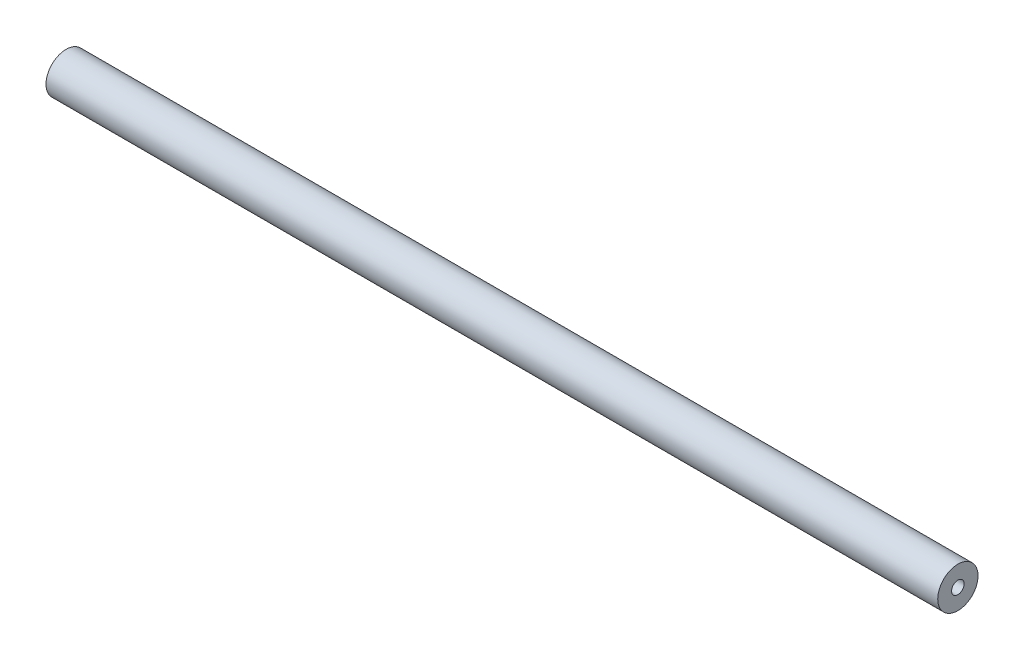
SolidWorks part; units mm, degrees
material "45"
ref_plane "Front" through (0, 0, 0) normal (0, 0, 1) x (1, 0, 0)
ref_plane "Top" through (0, 0, 0) normal (0, 1, 0) x (1, 0, 0)
ref_plane "Right" through (0, 0, 0) normal (1, 0, 0) x (0, 0, -1)
sketch "Sketch1" plane through (0, 0, 0) normal (0, 0, 1) x (1, 0, 0)
  line L0 (0, 0) -> (-177, 0) construction
  line L2 (177, 8) -> (-177, 8)
  line L6 (-177, 8) -> (-177, 0)
  line L7 (0, 0) -> (0, 8) construction
  line L8 (177, 8) -> (177, 0)
  line L13 (-177, 0) -> (177, 0)
  dimension "D1" = 354
  dimension "D5" = 8
revolve "Revolve1" add sketch "Sketch1" angle 360 about L13
hole_wizard "M6 Tapped Hole1" positions "Sketch2" profile "Sketch3" tap size "M6" standard "GB"
sketch "Sketch2" plane through (177, 0, 0) normal (1, 0, 0) x (0, 0, -1)
  point P0 (0, 0)
sketch "Sketch3" plane through (177, 0, 0) normal (0, 1, 0) x (0, 0, -1)
  line L0 (0, 0) -> (0, 16.5022)
  line L1 (0, 16.5022) -> (2.5, 15)
  line L2 (2.5, 15) -> (2.5, 0)
  line L5 (2.5, 0) -> (0, 0)
  line L10 (0, 16.5022) -> (-2.5, 15) construction
  line L11 (0, -6.35) -> (0, 107.95) construction
  dimension "螺纹孔钻头直径" = 5
  dimension "螺纹孔钻头深度" = 15
  dimension "导头角度" = 118
cosmetic thread "Cosmetic Thread1"
hole_wizard "M6 Tapped Hole2" positions "Sketch4" profile "Sketch5" tap size "M6" standard "GB"
sketch "Sketch4" plane through (-177, 0, 0) normal (-1, 0, 0) x (0, 0, 1)
  point P0 (0, 0)
sketch "Sketch5" plane through (-177, 0, 0) normal (0, 1, 0) x (0, 0, 1)
  line L0 (0, 0) -> (0, 16.5022)
  line L1 (0, 16.5022) -> (2.5, 15)
  line L2 (2.5, 15) -> (2.5, 0)
  line L5 (2.5, 0) -> (0, 0)
  line L10 (0, 16.5022) -> (-2.5, 15) construction
  line L11 (0, -6.35) -> (0, 107.95) construction
  dimension "螺纹孔钻头直径" = 5
  dimension "螺纹孔钻头深度" = 15
  dimension "导头角度" = 118
cosmetic thread "Cosmetic Thread2" parameters "D1"=12, "D2"=6
